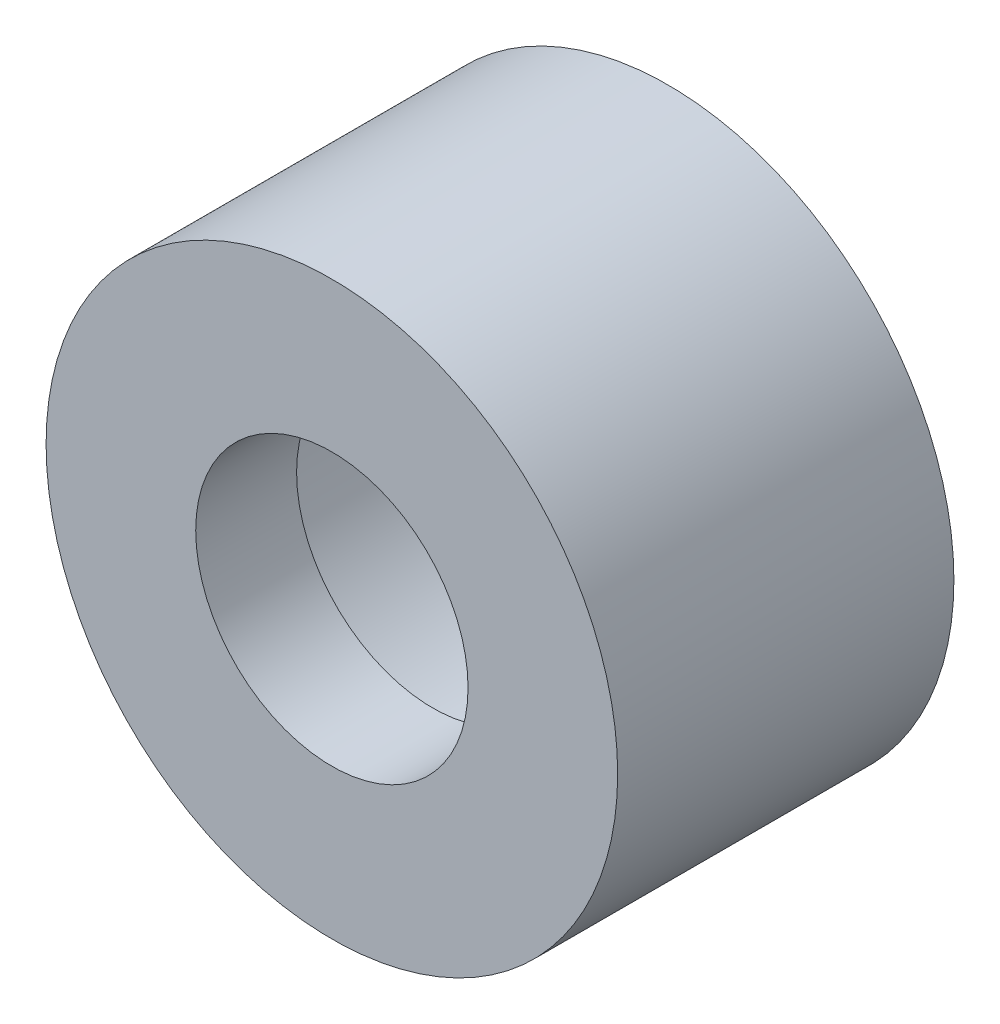
SolidWorks part; units mm, degrees
ref_plane "前视" through (0, 0, 0) normal (0, 0, 1) x (1, 0, 0)
ref_plane "上视" through (0, 0, 0) normal (0, 1, 0) x (1, 0, 0)
ref_plane "右视" through (0, 0, 0) normal (1, 0, 0) x (0, 0, -1)
sketch "草图1" plane through (0, 0, 0) normal (0, 0, 1) x (1, 0, 0)
  circle A0 centre (0, 0) radius 8.5
  circle A1 centre (0, 0) radius 4.05
  dimension "D1" = 8.1
  dimension "D2" = 17
extrude "凸台-拉伸1" add sketch "草图1" along normal blind 10
sketch "草图2" plane through (0, 0, 0) normal (0, 0, -1) x (-1, 0, 0)
  circle A0 centre (0, 0) radius 6.25
  dimension "D1" = 12.5
extrude "切除-拉伸1" cut sketch "草图2" against normal blind 7
